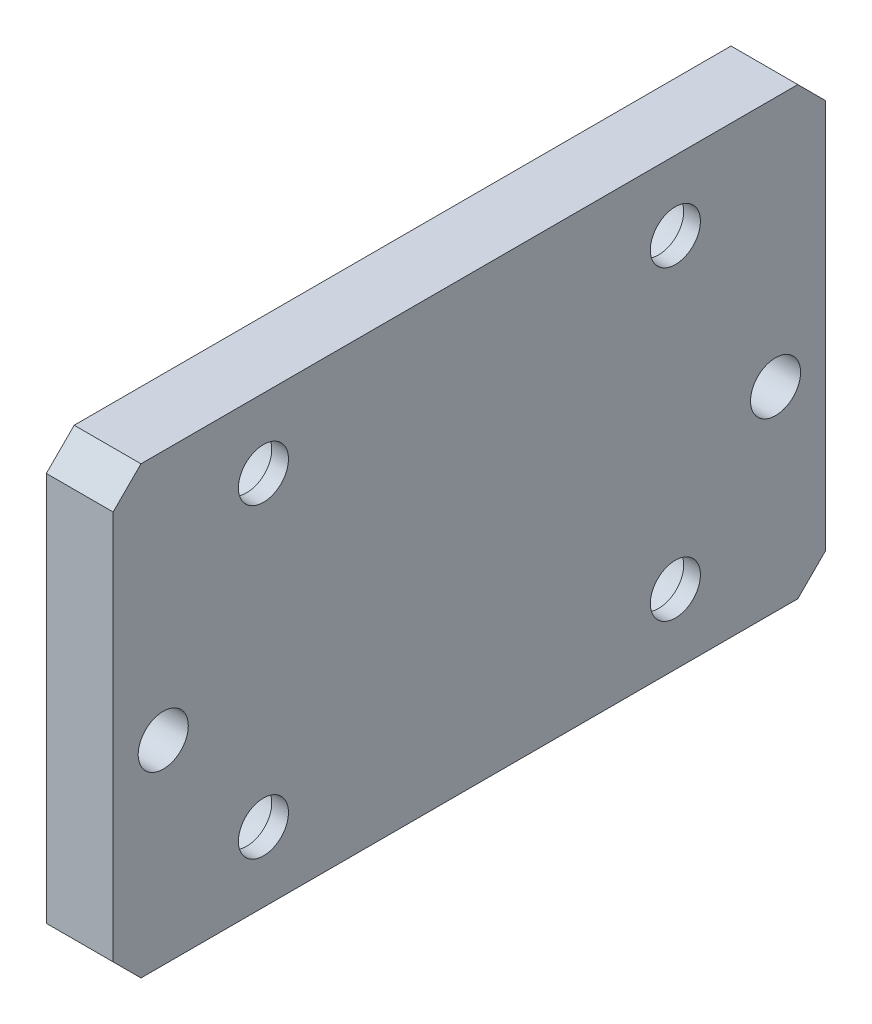
from build123d import *

# Parameters (mm, degrees)
SKETCH_1_W                = 128
SKETCH_1_H                = 80
EXTRUDE_1_DEPTH           = 12
HOLE_WIZARD_1_D           = 9
HOLE_WIZARD_1_CBORE_D     = 15
HOLE_WIZARD_1_CBORE_DEPTH = 9
HOLE_WIZARD_9_0_9_1_D     = 9
CHAMFER_1_SIZE            = 5


with BuildPart() as part:
    # 草图1 → 凸台-拉伸1 (new body)
    with BuildSketch(Plane(origin=(0, 0, 0), x_dir=(0, 0, -1), z_dir=(1, 0, 0))):
        Rectangle(SKETCH_1_W, SKETCH_1_H)
    extrude(amount=EXTRUDE_1_DEPTH)

    # 打孔尺寸(%根据)内六角圆柱头螺钉的类型1 (through all)
    with Locations(Plane.ZY):
        with Locations((-37, 27.5), (-37, -27.5), (37, 27.5), (37, -27.5)):
            CounterBoreHole(HOLE_WIZARD_1_D / 2, HOLE_WIZARD_1_CBORE_D / 2, HOLE_WIZARD_1_CBORE_DEPTH)

    # Ø9.0 (9) 直径孔1 (through all)
    with Locations(Plane(origin=(12, 0, 0), x_dir=(0, 0, -1), z_dir=(1, 0, 0))):
        with Locations((-55, -5), (55, -5)):
            Hole(HOLE_WIZARD_9_0_9_1_D / 2)

    # 倒角1
    chamfer_1_edges = [part.edges().sort_by_distance(p)[0] for p in [
        (6, -40, -64),
        (6, -40, 64),
        (6, 40, 64),
        (6, 40, -64),
    ]]
    chamfer(chamfer_1_edges, length=CHAMFER_1_SIZE)


solid = part.part
